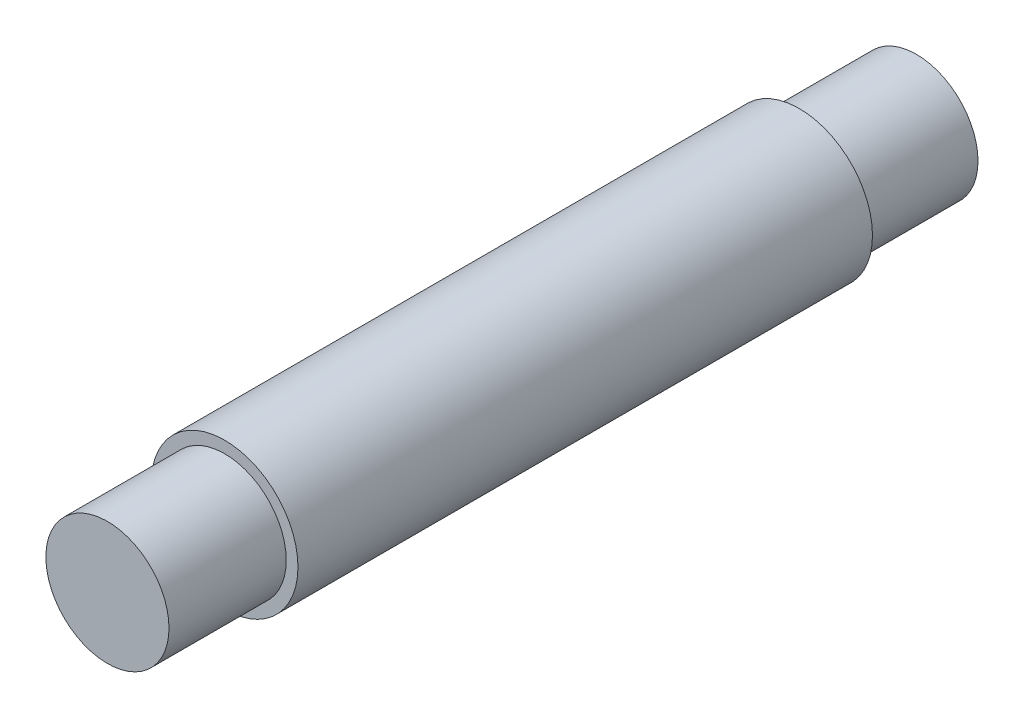
SolidWorks part; units mm, degrees
ref_plane "Front Plane" through (0, 0, 0) normal (0, 0, 1) x (1, 0, 0)
ref_plane "Top Plane" through (0, 0, 0) normal (0, 1, 0) x (1, 0, 0)
ref_plane "Right Plane" through (0, 0, 0) normal (1, 0, 0) x (0, 0, -1)
sketch "Sketch 1" plane through (0, 0, 0) normal (0, 0, 1) x (1, 0, 0)
  line L0 (0, 55.4084) -> (0, -50.1461) construction
  line L1 (-164.9606, 0) -> (173.305, 0) construction
  circle A0 centre (0, 0) radius 25
  dimension "D1" = 50
extrude "Boss-Extrude 1" add sketch "Sketch 1" along normal mid plane 196
sketch "Sketch 2" plane through (0, 0, 98) normal (0, 0, 1) x (1, 0, 0)
  circle A0 centre (0, 0) radius 21
  dimension "D1" = 42
extrude "Boss-Extrude 2" add sketch "Sketch 2" along normal blind 40
mirror "Mirror 1" about plane through (0, 0, 0) normal (0, 0, 1) of "Boss-Extrude 2"
